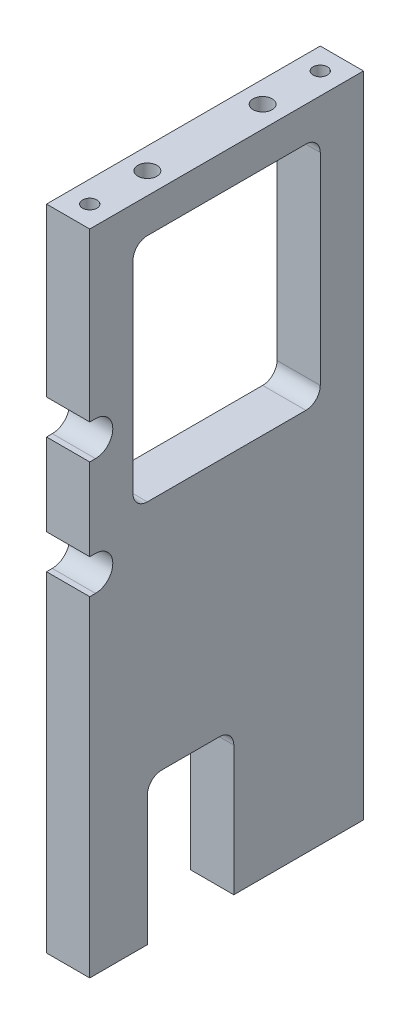
SolidWorks part; units mm, degrees
material "A6061"
ref_plane "Front Plane" through (0, 0, 0) normal (0, 0, 1) x (1, 0, 0)
ref_plane "Top Plane" through (0, 0, 0) normal (0, 1, 0) x (1, 0, 0)
ref_plane "Right Plane" through (0, 0, 0) normal (1, 0, 0) x (0, 0, -1)
sketch "Sketch1" plane through (0, 0, 0) normal (1, 0, 0) x (0, 0, -1)
  line L1 (-47.5, -112.55) -> (47.5, -112.55)
  line L2 (-47.5, -112.55) -> (-47.5, 112.55)
  line L3 (-47.5, 112.55) -> (47.5, 112.55)
  line L4 (47.5, -112.55) -> (47.5, 112.55)
  line L5 (-47.5, -112.55) -> (47.5, 112.55) construction
  line L6 (-47.5, 112.55) -> (47.5, -112.55) construction
  point P0 (0, 0)
  dimension "D1" = 95
  dimension "D2" = 225.1
extrude "Boss-Extrude1" add sketch "Sketch1" along normal blind 15
sketch "Sketch2" plane through (0, 0, 0) normal (-1, 0, 0) x (0, 0, 1)
  line L0 (-47.5, -112.55) -> (-47.5, 112.55) construction
  line L1 (47.5, -112.55) -> (-47.5, -112.55) construction
  line L2 (22.5, -62.55) -> (2.5, -62.55)
  line L3 (27.5, -67.55) -> (27.5, -112.55)
  line L4 (27.5, -112.55) -> (-2.5, -112.55)
  line L5 (-2.5, -67.55) -> (-2.5, -112.55)
  line L6 (27.5, -62.55) -> (-2.5, -112.55) construction
  line L7 (27.5, -112.55) -> (-2.5, -62.55) construction
  line L8 (47.5, 112.55) -> (47.5, -112.55) construction
  line L9 (-27.5, 20.55) -> (27.5, 20.55)
  line L10 (-32.5, 25.55) -> (-32.5, 95.55)
  line L11 (-27.5, 100.55) -> (27.5, 100.55)
  line L12 (32.5, 25.55) -> (32.5, 95.55)
  line L13 (-32.5, 20.55) -> (32.5, 100.55) construction
  line L14 (-32.5, 100.55) -> (32.5, 20.55) construction
  line L15 (-47.5, 112.55) -> (47.5, 112.55) construction
  arc A0 (22.5, -62.55) -> (27.5, -67.55) centre (22.5, -67.55) cw
  arc A1 (2.5, -62.55) -> (-2.5, -67.55) centre (2.5, -67.55) ccw
  arc A2 (27.5, 20.55) -> (32.5, 25.55) centre (27.5, 25.55) ccw
  arc A3 (-27.5, 20.55) -> (-32.5, 25.55) centre (-27.5, 25.55) cw
  arc A4 (27.5, 100.55) -> (32.5, 95.55) centre (27.5, 95.55) cw
  arc A5 (-32.5, 95.55) -> (-27.5, 100.55) centre (-27.5, 95.55) cw
  point P3 (12.5, -87.55)
  point P16 (0, 60.55)
  dimension "D3" = 5
  dimension "D7" = 5
  dimension "D1" = 30
  dimension "D2" = 50
  dimension "D4" = 15
  dimension "D5" = 12
  dimension "D6" = 80
  dimension "D8" = 20
  dimension "D9" = 15
extrude "Cut-Extrude1" cut sketch "Sketch2" against normal through all
hole_wizard "M6 Clearance Hole1" positions "Sketch6" profile "Sketch7" hole size "M6" standard "GB"
sketch "Sketch6" plane through (0, 112.55, 0) normal (0, 1, 0) x (1, 0, 0)
  line L0 (0, 0) -> (15, 0) construction
  line L1 (15, 47.5) -> (15, -47.5) construction
  line L3 (7.5, 47.5) -> (7.5, -47.5) construction
  line L4 (15, 47.5) -> (0, 47.5) construction
  line L5 (15, -47.5) -> (0, -47.5) construction
  point P16 (7.5, 20)
  point P18 (7.5, -20)
  dimension "D1" = 40
sketch "Sketch7" plane through (7.5, 112.55, 20) normal (1, 0, 0) x (0, 0, 1)
  line L0 (0, 0) -> (0, 21.7328)
  line L1 (0, 21.7328) -> (3.3, 19.75)
  line L2 (3.3, 19.75) -> (3.3, 0)
  line L5 (3.3, 0) -> (0, 0)
  line L10 (0, 21.7328) -> (-3.3, 19.75) construction
  line L11 (0, -6.35) -> (0, 107.95) construction
  dimension "孔直径" = 6.6
  dimension "孔深度" = 19.75
  dimension "导头角度" = 118
hole_wizard "M6 Tapped Hole1" positions "Sketch8" profile "Sketch9" tap size "M6" standard "GB"
sketch "Sketch8" plane through (0, -112.55, 0) normal (0, -1, 0) x (-1, 0, 0)
  line L0 (0, 0) -> (-15, 0) construction
  line L3 (-7.5, 47.5) -> (-7.5, -47.5) construction
  line L4 (-15, 47.5) -> (0, 47.5) construction
  line L5 (-15, -47.5) -> (0, -47.5) construction
  line L6 (-15, 2.5) -> (-15, 47.5) construction
  point P16 (-7.5, 40)
  point P18 (-7.5, -40)
  dimension "D1" = 80
sketch "Sketch9" plane through (7.5, -112.55, 40) normal (1, 0, 0) x (0, 0, -1)
  line L0 (0, 0) -> (0, 16.5022)
  line L1 (0, 16.5022) -> (2.5, 15)
  line L2 (2.5, 15) -> (2.5, 0)
  line L5 (2.5, 0) -> (0, 0)
  line L10 (0, 16.5022) -> (-2.5, 15) construction
  line L11 (0, -6.35) -> (0, 107.95) construction
  dimension "螺纹孔钻头直径" = 5
  dimension "螺纹孔钻头深度" = 15
  dimension "导头角度" = 118
hole_wizard "Ø5.0mm blind hole 1" positions "Sketch10" profile "Sketch11" hole size "Ø5.0" standard "GB"
sketch "Sketch10" plane through (0, -112.55, 0) normal (0, -1, 0) x (-1, 0, 0)
  line L0 (-7.5, 40) -> (-7.5, -40) construction
  point P7 (-7.5, 10)
  dimension "D1" = 10
sketch "Sketch11" plane through (7.5, -112.55, -10) normal (1, 0, 0) x (0, 0, -1)
  line L0 (0, 0) -> (0, 9.5022)
  line L1 (0, 9.5022) -> (2.5, 8)
  line L2 (2.5, 8) -> (2.5, 0)
  line L5 (2.5, 0) -> (0, 0)
  line L10 (0, 9.5022) -> (-2.5, 8) construction
  line L11 (0, -6.35) -> (0, 107.95) construction
  dimension "孔直径" = 5
  dimension "孔深度" = 8
  dimension "导头角度" = 118
hole_wizard "Ø5.0mm blind hole 2" positions "Sketch12" profile "Sketch13" hole size "Ø5.0" standard "GB"
sketch "Sketch12" plane through (0, 112.55, 0) normal (0, 1, 0) x (1, 0, 0)
  line L0 (0, 0) -> (15, 0) construction
  line L1 (15, 47.5) -> (15, -47.5) construction
  line L3 (7.5, 47.5) -> (7.5, -47.5) construction
  line L4 (15, 47.5) -> (0, 47.5) construction
  line L5 (15, -47.5) -> (0, -47.5) construction
  point P16 (7.5, 40)
  point P18 (7.5, -40)
  dimension "D1" = 80
sketch "Sketch13" plane through (7.5, 112.55, 40) normal (1, 0, 0) x (0, 0, 1)
  line L0 (0, 0) -> (0, 9.5022)
  line L1 (0, 9.5022) -> (2.5, 8)
  line L2 (2.5, 8) -> (2.5, 0)
  line L5 (2.5, 0) -> (0, 0)
  line L10 (0, 9.5022) -> (-2.5, 8) construction
  line L11 (0, -6.35) -> (0, 107.95) construction
  dimension "孔直径" = 5
  dimension "孔深度" = 8
  dimension "导头角度" = 118
sketch "Sketch14" plane through (15, 0, 0) normal (1, 0, 0) x (0, 0, -1)
  circle A0 centre (-45.5, 48.55) radius 6
  circle A1 centre (-45.5, 8.05) radius 6
  dimension "D1" = 12
extrude "Cut-Extrude2" cut sketch "Sketch14" against normal through all
sketch "Sketch15" plane through (0, 0, 0) normal (-1, 0, 0) x (0, 0, 1)
  line L0 (45.5, 8.05) -> (64.1978, 8.05) construction
  line L1 (45.5, 48.55) -> (74.3381, 48.55) construction
  line L6 (55.5, 2.05) -> (45.5, 2.05)
  line L7 (55.5, 2.05) -> (55.5, 14.05)
  line L8 (55.5, 14.05) -> (45.5, 14.05)
  line L9 (45.5, 2.05) -> (45.5, 14.05)
  line L10 (55.5, 2.05) -> (45.5, 14.05) construction
  line L11 (55.5, 14.05) -> (45.5, 2.05) construction
  line L13 (55.5, 42.55) -> (45.5, 42.55)
  line L14 (55.5, 42.55) -> (55.5, 54.55)
  line L15 (55.5, 54.55) -> (45.5, 54.55)
  line L16 (45.5, 42.55) -> (45.5, 54.55)
  line L17 (55.5, 42.55) -> (45.5, 54.55) construction
  line L18 (55.5, 54.55) -> (45.5, 42.55) construction
  arc A1 (47.5, 13.7069) -> (47.5, 2.3931) centre (45.5, 8.05) ccw construction
  arc A2 (47.5, 54.2069) -> (47.5, 42.8931) centre (45.5, 48.55) ccw construction
  point P3 (50.5, 8.05)
  point P15 (50.5, 48.55)
  dimension "D1" = 10
extrude "Cut-Extrude3" cut sketch "Sketch15" against normal through all
hole_wizard "M5 Tapped Hole1" positions "Sketch18" profile "Sketch19" tap size "M5" standard "GB"
sketch "Sketch18" plane through (0, 0, 0) normal (-1, 0, 0) x (0, 0, 1)
  line L0 (-47.5, 112.55) -> (47.5, 112.55) construction
  line L1 (-47.5, -112.55) -> (-47.5, 112.55) construction
  point P0 (-40, -77.45)
  point P2 (-40, 67.55)
  dimension "D1" = 45
  dimension "D2" = 145
  dimension "D3" = 7.5
sketch "Sketch19" plane through (0, -77.45, -40) normal (0, 1, 0) x (0, 0, 1)
  line L0 (0, 0) -> (0, 13.6618)
  line L1 (0, 13.6618) -> (2.1, 12.4)
  line L2 (2.1, 12.4) -> (2.1, 0)
  line L5 (2.1, 0) -> (0, 0)
  line L10 (0, 13.6618) -> (-2.1, 12.4) construction
  line L11 (0, -6.35) -> (0, 107.95) construction
  dimension "螺纹孔钻头直径" = 4.2
  dimension "螺纹孔钻头深度" = 12.4
  dimension "导头角度" = 118
mirror "Mirror1" about plane through (0, 0, 0) normal (0, 0, 1) of "M5 Tapped Hole1"
